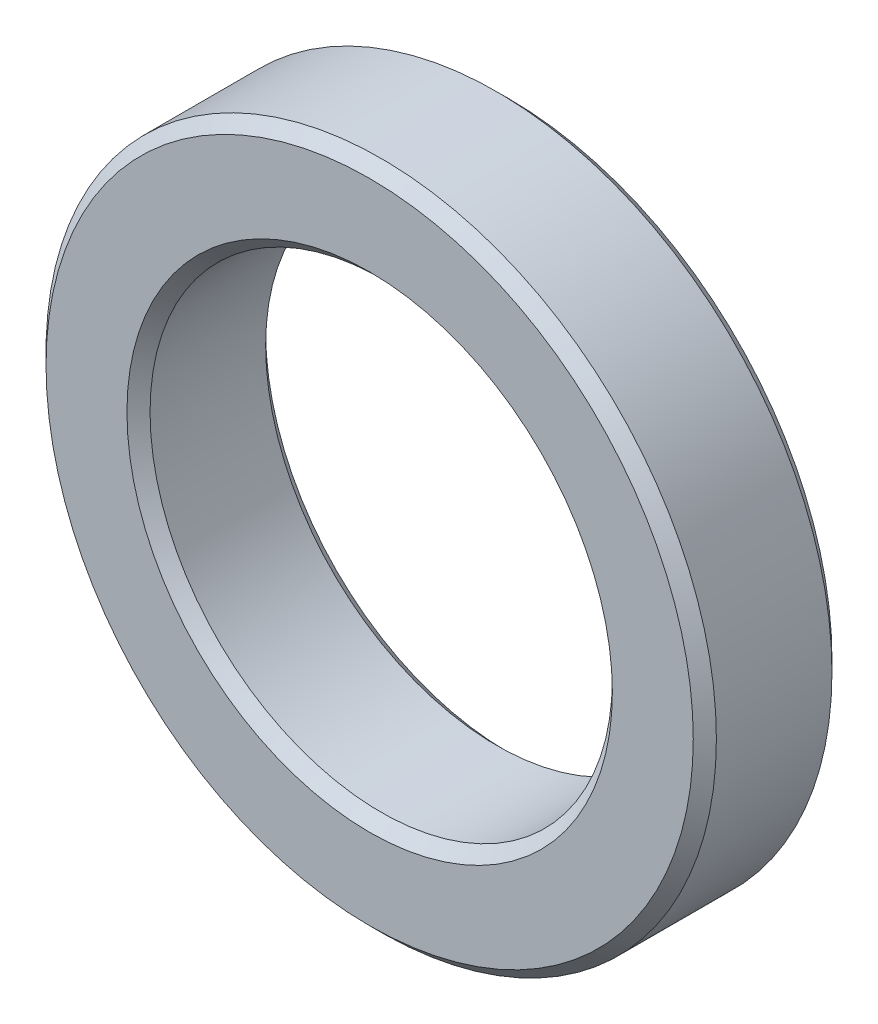
SolidWorks part; units mm, degrees
material "SUS 303"
ref_plane "Front Plane" through (0, 0, 0) normal (0, 0, 1) x (1, 0, 0)
ref_plane "Top Plane" through (0, 0, 0) normal (0, 1, 0) x (1, 0, 0)
ref_plane "Right Plane" through (0, 0, 0) normal (1, 0, 0) x (0, 0, -1)
sketch "Sketch1" plane through (0, 0, 0) normal (0, 1, 0) x (1, 0, 0)
  line L0 (0, 0) -> (0, 1.8396) construction
  line L1 (2.1, 0) -> (2.8, 0)
  line L2 (2, 0.1) -> (2, 1.1)
  line L3 (2.1, 1.2) -> (2.8, 1.2)
  line L4 (2.9, 0.1) -> (2.9, 1.1)
  line L5 (2, 0.1) -> (2.1, 0)
  line L6 (2.8, 0) -> (2.9, 0.1)
  line L7 (2.8, 1.2) -> (2.9, 1.1)
  line L8 (2, 1.1) -> (2.1, 1.2)
  point P0 (2, 0)
  point P1 (2.9, 1.2)
  point P2 (2, 1.2)
  point P3 (2.9, 0)
  dimension "D1" = 4
  dimension "D2" = 5.8
  dimension "D3" = 1.2
revolve "Revolve1" add sketch "Sketch1" angle 360 about L0
